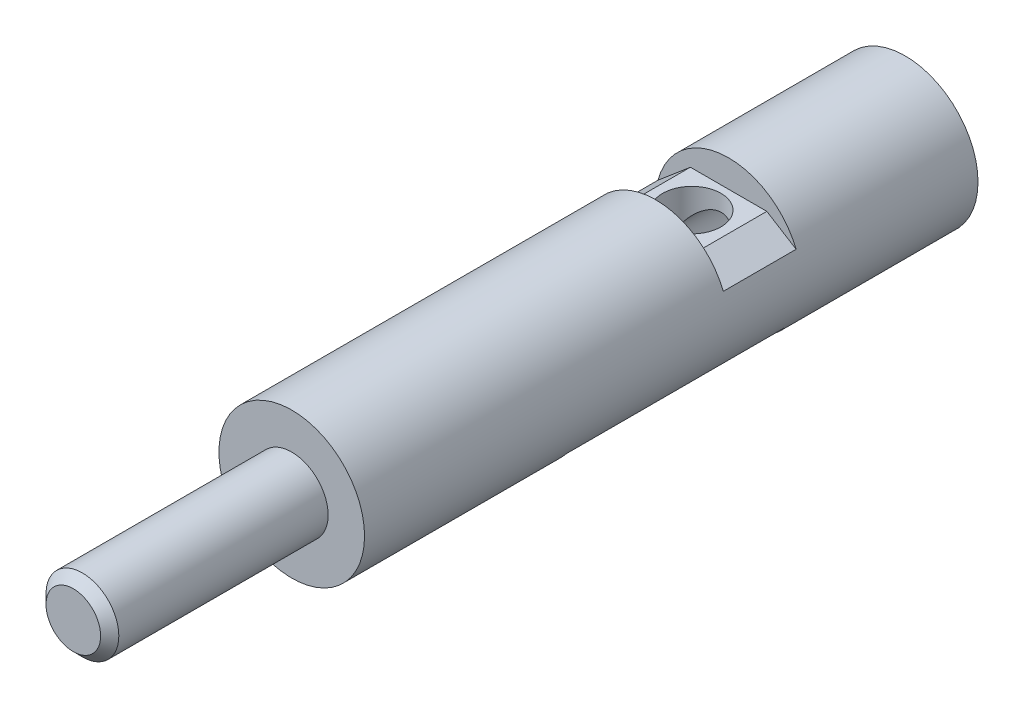
from build123d import *
from build123d.topology import SkipClean

# Parameters (mm, degrees)
SKETCH_1_2_R                   = 4
BOSS_EXTRUDE1_DEPTH            = 9.7
BOSS_EXTRUDE2_DEPTH            = 4
BOSS_EXTRUDE3_START            = 13.7
SKETCH_1_2_2_R                 = 4
BOSS_EXTRUDE3_DEPTH            = 20
SKETCH3_R                      = 2
BOSS_EXTRUDE4_DEPTH            = 12
CHAMFER1_SIZE                  = 0.5
CUT_EXTRUDE1_DEPTH             = 12
F_3_2_3_2_DIAMETER_HOLE1_D     = 3.2
F_3_2_3_2_DIAMETER_HOLE1_DEPTH = 14
F_3_2_3_2_DIAMETER_HOLE1_TIP   = 0.96137699
F_3_2_3_2_DIAMETER_HOLE2_D     = 3.2
F_3_2_3_2_DIAMETER_HOLE2_DEPTH = 2.499
F_3_2_3_2_DIAMETER_HOLE2_TIP   = 0.96137699


with BuildPart() as part:
    # Sketch 1_2 → Boss-Extrude1 (new body)
    with BuildSketch(Plane.XY):
        Circle(SKETCH_1_2_R)
    extrude(amount=BOSS_EXTRUDE1_DEPTH)

    # Sketch2 → Boss-Extrude2 (add)
    with SkipClean():  # the faces are left unmerged after this step: merging them gives an invalid solid
        with BuildSketch(Plane.XY.offset(9.7)):
            with BuildLine():
                Line((-3.872983346, 1), (-2.1, 2.5))
                Line((-2.1, 2.5), (2.1, 2.5))
                Line((2.1, 2.5), (3.708099244, 1.5))
                ThreePointArc((3.708099244, 1.5), (3.957811022, -0.579423775), (3.122498999, -2.5))
                Line((3.122498999, -2.5), (-3.122498999, -2.5))
                ThreePointArc((-3.122498999, -2.5), (-3.911098735, -0.838633823), (-3.872983346, 1))
            make_face()
        extrude(amount=BOSS_EXTRUDE2_DEPTH)

    # Sketch 1_2 2 → Boss-Extrude3 (add)
    with SkipClean():  # the faces are left unmerged after this step: merging them gives an invalid solid
        with BuildSketch(Plane.XY.offset(BOSS_EXTRUDE3_START)):
            Circle(SKETCH_1_2_2_R)
        extrude(amount=BOSS_EXTRUDE3_DEPTH)

    # Sketch3 → Boss-Extrude4 (add)
    with SkipClean():  # the faces are left unmerged after this step: merging them gives an invalid solid
        with BuildSketch(Plane.XY.offset(33.7)):
            Circle(SKETCH3_R)
        extrude(amount=BOSS_EXTRUDE4_DEPTH)

    # Chamfer1
    chamfer1_edges = [part.edges().sort_by_distance(p)[0] for p in [
        (-2, 0, 45.7),
    ]]
    chamfer(chamfer1_edges, length=CHAMFER1_SIZE)

    # Sketch4 → Cut-Extrude1 (cut)
    with SkipClean():  # the faces are left unmerged after this step: merging them gives an invalid solid
        with BuildSketch(Plane.XY.offset(9.7)):
            with BuildLine():
                Line((3.122498999, -2.5), (-3.122498999, -2.5))
                ThreePointArc((-3.122498999, -2.5), (0, -4), (3.122498999, -2.5))
            make_face()
        extrude(amount=CUT_EXTRUDE1_DEPTH, mode=Mode.SUBTRACT)

    # Ø3.2 (3.2) Diameter Hole1
    with Locations(Plane(origin=(0, 0, 0), x_dir=(-1, 0, 0), z_dir=(0, 0, -1))):
        with Locations((0, 0)):
            Hole(F_3_2_3_2_DIAMETER_HOLE1_D / 2, depth=F_3_2_3_2_DIAMETER_HOLE1_DEPTH)
            with Locations((0, 0, -(F_3_2_3_2_DIAMETER_HOLE1_DEPTH + F_3_2_3_2_DIAMETER_HOLE1_TIP / 2))):  # 118° drill point
                Cone(0, F_3_2_3_2_DIAMETER_HOLE1_D / 2, F_3_2_3_2_DIAMETER_HOLE1_TIP, mode=Mode.SUBTRACT)

    # Ø3.2 (3.2) Diameter Hole2
    with Locations(Plane(origin=(-0.020216214, 2.5, 11.7), x_dir=(0, 0, 1), z_dir=(0, 1, 0))):
        with Locations((0, 0)):
            Hole(F_3_2_3_2_DIAMETER_HOLE2_D / 2, depth=F_3_2_3_2_DIAMETER_HOLE2_DEPTH)
            with Locations((0, 0, -(F_3_2_3_2_DIAMETER_HOLE2_DEPTH + F_3_2_3_2_DIAMETER_HOLE2_TIP / 2))):  # 118° drill point
                Cone(0, F_3_2_3_2_DIAMETER_HOLE2_D / 2, F_3_2_3_2_DIAMETER_HOLE2_TIP, mode=Mode.SUBTRACT)


solid = part.part
